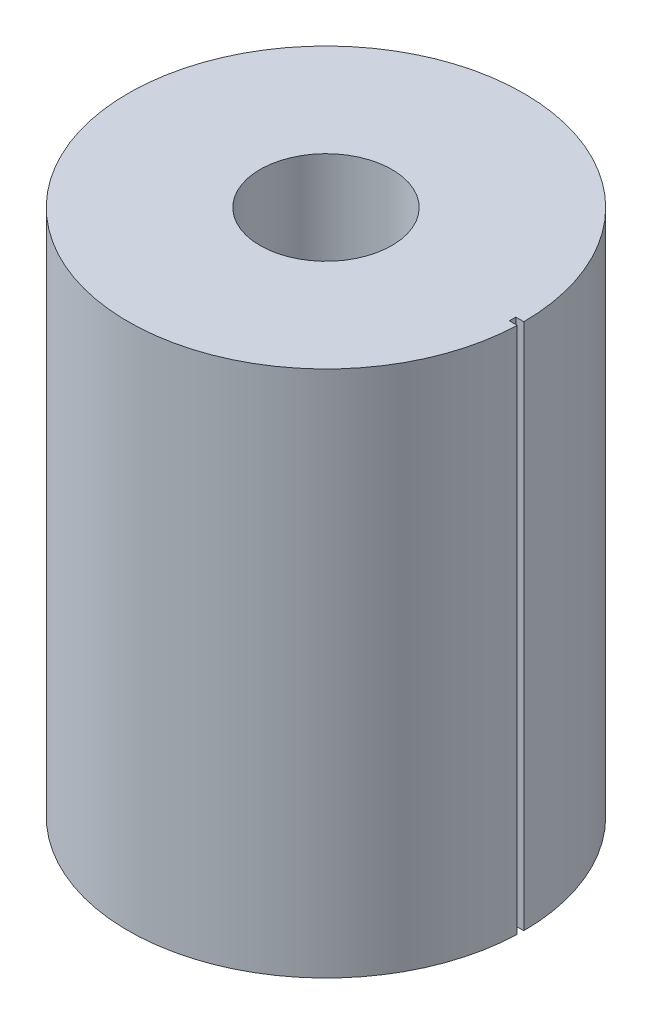
from build123d import *

# Parameters (mm, degrees)
SKETCH1_R           = 7.5
SKETCH1_R_2         = 2.5
BOSS_EXTRUDE1_DEPTH = 20
SKETCH2_W           = 0.602620298
SKETCH2_H           = 0.245198841
CUT_EXTRUDE1_DEPTH  = 23.638462845


with BuildPart() as part:
    # Sketch1 → Boss-Extrude1 (new body)
    with BuildSketch(Plane(origin=(0, 0, 0), x_dir=(1, 0, 0), z_dir=(0, 1, 0))):
        with Locations(Location((0, 0, 0), (0, 0, 270))):
            Circle(SKETCH1_R)
        with Locations(Location((0, 0, 0), (0, 0, 270))):
            Circle(SKETCH1_R_2, mode=Mode.SUBTRACT)
    extrude(amount=BOSS_EXTRUDE1_DEPTH)

    # Sketch2 → Cut-Extrude1 (cut, through all)
    with BuildSketch(Plane(origin=(0, 20, 0), x_dir=(1, 0, 0), z_dir=(0, 1, 0))):
        with Locations((7.498997892, -0.122599421)):
            Rectangle(SKETCH2_W, SKETCH2_H)
    extrude(amount=-CUT_EXTRUDE1_DEPTH, mode=Mode.SUBTRACT)


solid = part.part
